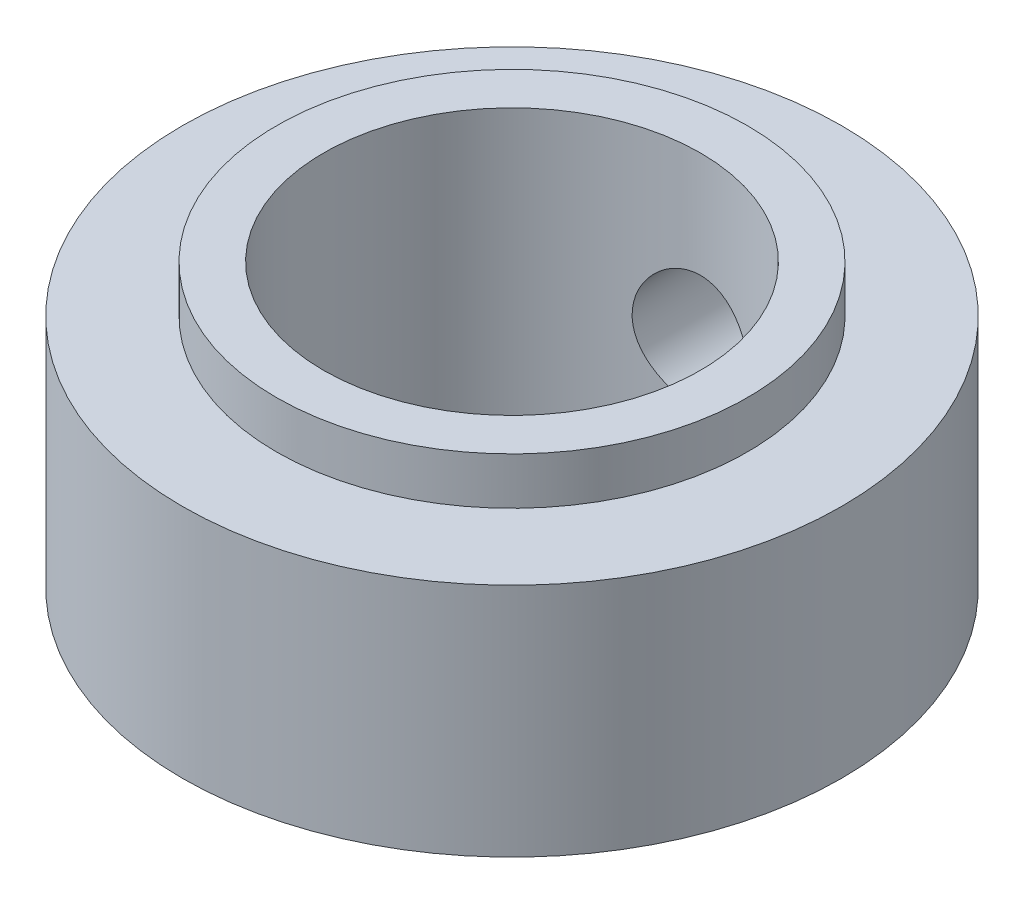
from build123d import *

# Parameters (mm, degrees)
SKETCH_2_R          = 1.25
CUT_EXTRUDE_1_DEPTH = 10


with BuildPart() as part:
    # 草图1 → 旋转1 (revolve)
    with BuildSketch(Plane.XY, mode=Mode.PRIVATE) as revolve_1_sk:
        Polygon((4, 4.368271468), (5, 4.368271468), (5, 3.368271468), (7, 3.368271468), (7, -1.631728532), (4, -1.631728532), align=None)
    revolve(revolve_1_sk.sketch.rotate(Axis((0, 0, 0), (0, 1, 0)), 90), axis=Axis((0, 0, 0), (0, 1, 0)))

    # 草图2 → 切除-拉伸1 (cut)
    with BuildSketch(Plane.XY):
        with Locations(Location((0, 0.868271468, 0), (0, 0, 270.000000001))):
            Circle(SKETCH_2_R)
    extrude(amount=-CUT_EXTRUDE_1_DEPTH, mode=Mode.SUBTRACT)


solid = part.part
